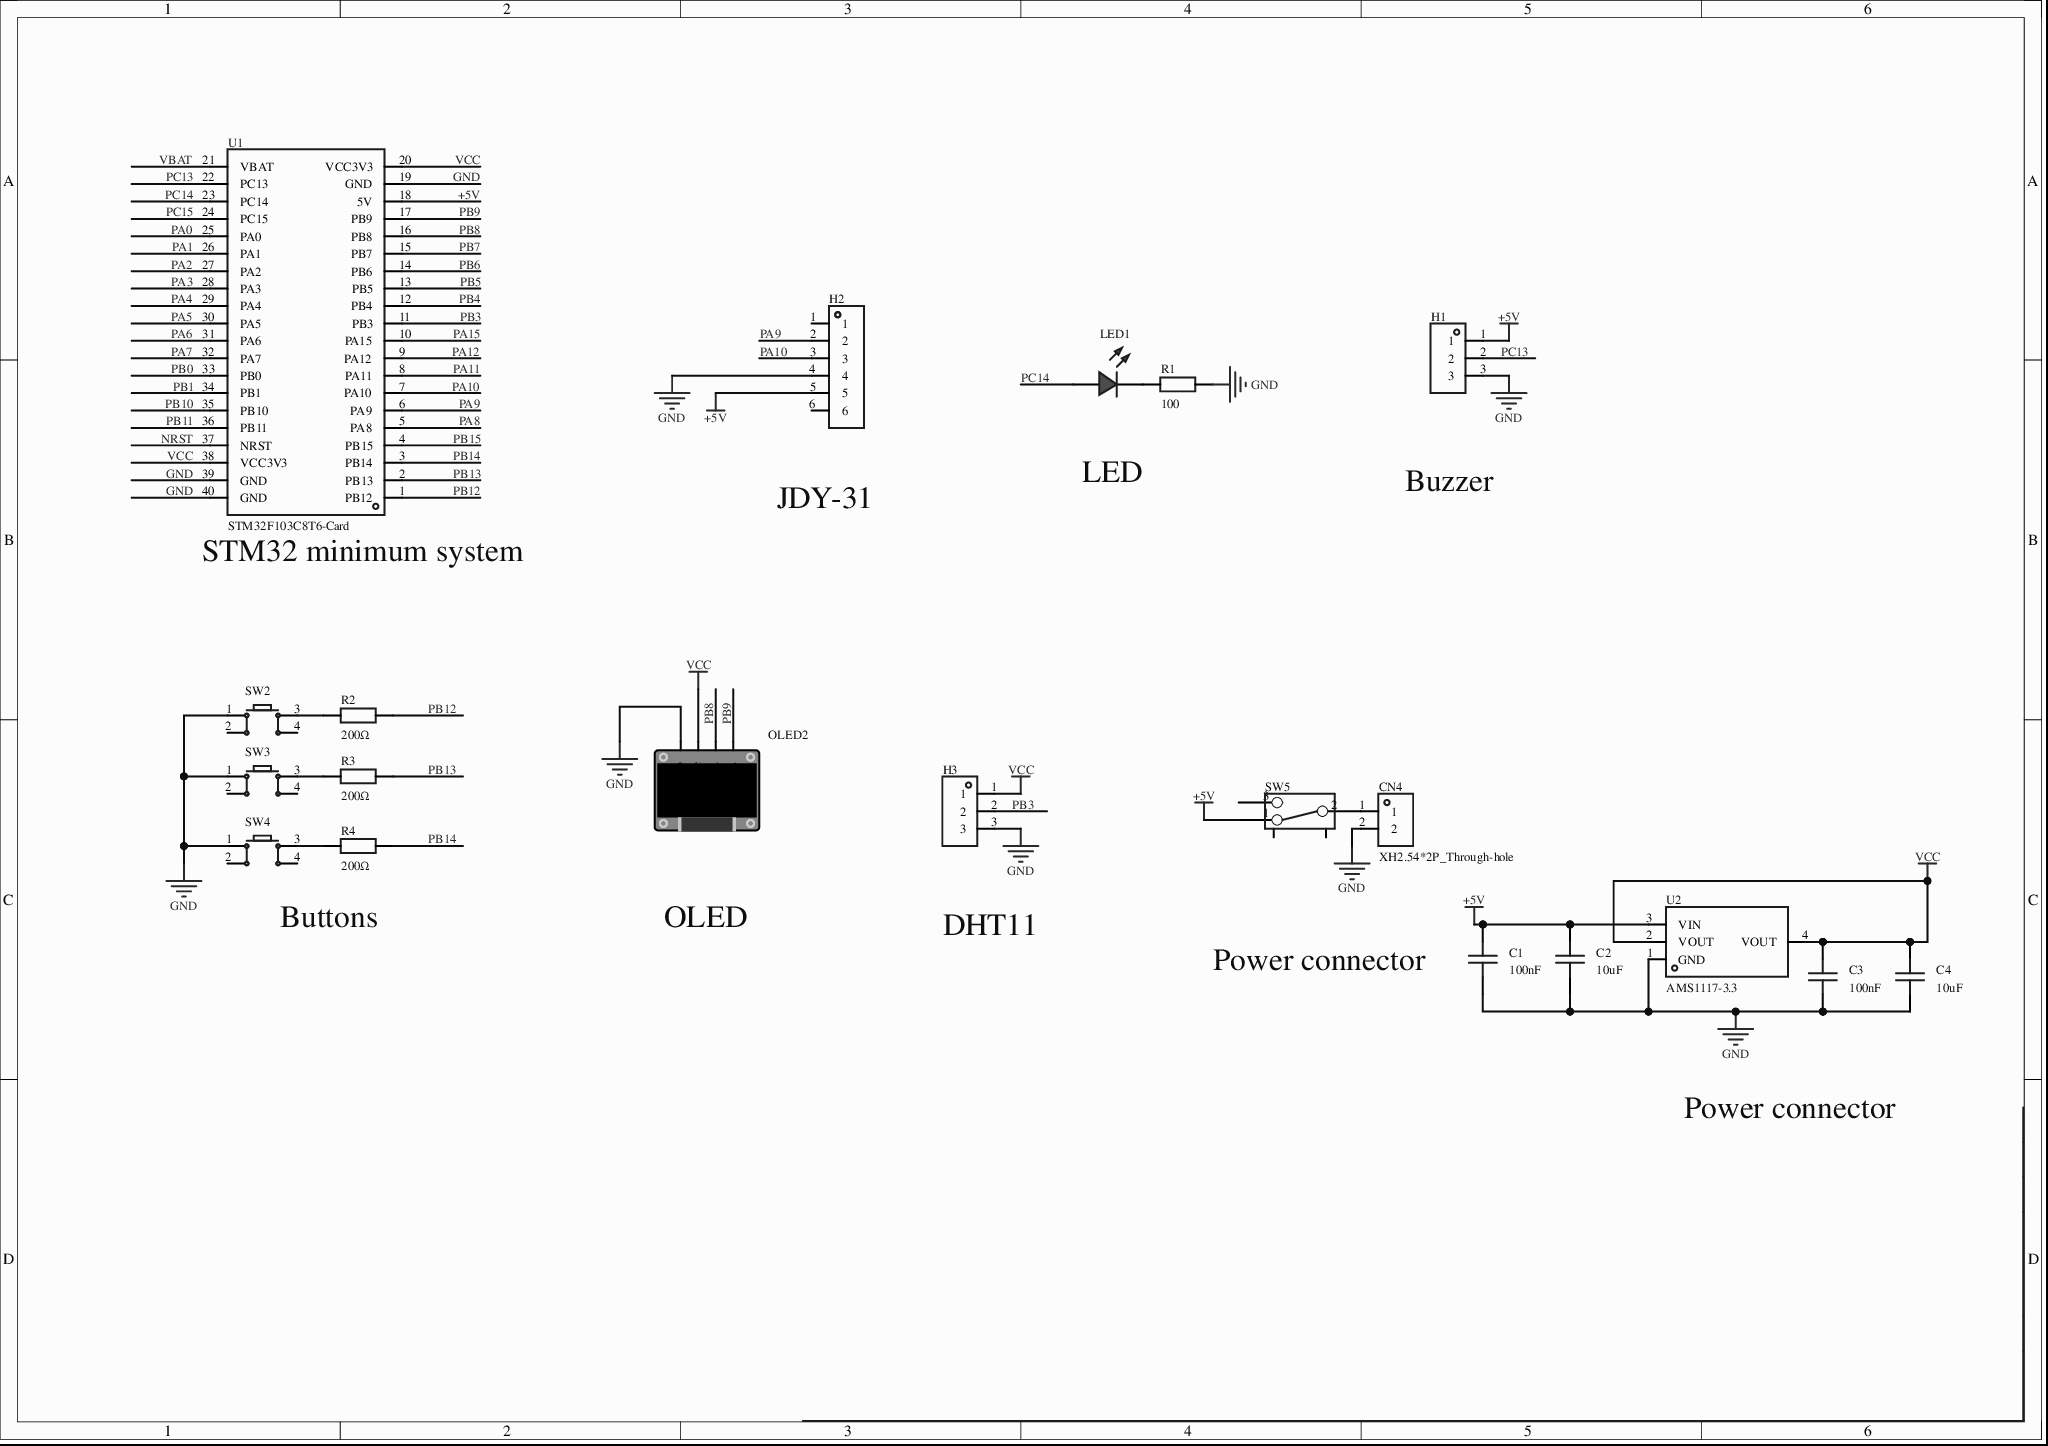
[diagram p0: MISC51821-3.schdoc]
# Altium project MISC51821-2.PrjPcb
1 sheet, 20 parts. Net scope: global (net labels, ports and power ports of the same name join across sheets).
Board file: MISC51821.pcbdoc

## Sheet MISC51821-3.schdoc
size 297 x 209 mm; Version: V1.0; @Project Name: MISC51821; @Page Count: 1; @Update Date: 2026-04-25; @Create Date: 2026-04-25; @Schematic Name: MISC51821; @Page No: 1; @Create Time: 23:22:16; @Update Time: 17:32:40; @Board Name: MISC51821

### Parts
C1  100nF  [C0603]
C2  10uF  [C0603]
C3  100nF  [C0603]
C4  10uF  [C0603]
CN4  XH2.54*2P_Through-hole  [CONN-TH_2P-P2.50-XH2.54-2P]
H1  (no value)  [HDR-TH_3P-P2.54-V-F]
H2  (no value)  [HDR-TH_6P-P2.54-V-F]
H3  (no value)  [HDR-TH_3P-P2.54-V-F]
LED1  (no value)  [LED_TH-3mm]
OLED2  (no value)  [0.96OLED_4P]
R1  100  [Res_1/8W]
R2  200Ω  [Res_1/8W]
R3  200Ω  [Res_1/8W]
R4  200Ω  [Res_1/8W]
SW2  (no value)  [SW-TH_4P-L6.0-W6.0-P4.50-LS6.5]
SW3  (no value)  [SW-TH_4P-L6.0-W6.0-P4.50-LS6.5]
SW4  (no value)  [SW-TH_4P-L6.0-W6.0-P4.50-LS6.5]
SW5  (no value)  [拨动开关]
U1  STM32F103C8T6-Card  [CONN-TH_L53.3-W22.9_STM32F103C8T6-CARD]
U2  AMS1117-3.3  [SOT-223-3_L6.5-W3.4-P2.30-LS7.0-BR]

### Nets
+5V: C1.2 C2.2 H1.1 H2.5 SW5.1 U1.18(5V) U2.3(VIN)
GND: C1.1 C2.1 C3.1 C4.1 CN4.2 H1.3 H2.4 H3.3 OLED2.1(GND) R1.2 SW2.1 SW3.1 SW4.1 U1.19(GND) U1.39(GND) U1.40(GND) U2.1(GND)
VCC: C3.2 C4.2 H3.1 OLED2.2(VCC) U1.20(VCC3V3) U1.38(VCC3V3) U2.2(VOUT) U2.4(VOUT)
NRST: U1.37(NRST)
PA0: U1.25(PA0)
PA1: U1.26(PA1)
PA2: U1.27(PA2)
PA3: U1.28(PA3)
PA4: U1.29(PA4)
PA5: U1.30(PA5)
PA6: U1.31(PA6)
PA7: U1.32(PA7)
PA8: U1.5(PA8)
PA9: H2.2 U1.6(PA9)
PA10: H2.3 U1.7(PA10)
PA11: U1.8(PA11)
PA12: U1.9(PA12)
PA15: U1.10(PA15)
PB0: U1.33(PB0)
PB1: U1.34(PB1)
PB3: H3.2 U1.11(PB3)
PB4: U1.12(PB4)
PB5: U1.13(PB5)
PB6: U1.14(PB6)
PB7: U1.15(PB7)
PB8: OLED2.3(SCL) U1.16(PB8)
PB9: OLED2.4(SDA) U1.17(PB9)
PB10: U1.35(PB10)
PB11: U1.36(PB11)
PB12: R2.2 U1.1(PB12)
PB13: R3.2 U1.2(PB13)
PB14: R4.2 U1.3(PB14)
PB15: U1.4(PB15)
PC13: H1.2 U1.22(PC13)
PC14: LED1.1(C) U1.23(PC14)
PC15: U1.24(PC15)
VBAT: U1.21(VBAT)
NetCN4_1: CN4.1 SW5.2
NetLED1_2: LED1.2(A) R1.1
NetR2_1: R2.1 SW2.3
NetR3_1: R3.1 SW3.3
NetR4_1: R4.1 SW4.3

Not connected (* = marked no-connect by the designer): H2 1 6; SW2 2 4; SW3 2 4; SW4 2 4; SW5 3 4 5

### Notes on the sheet
- 主控：
  STM32F103C8T6
  晶振电路
  复位电路
  串口：
  JDY-31  		PA9，PA10 	(串口1）
  GPIO:
  LED灯	PC14
  蜂鸣器  PC13
  按键：	PB12设置键，PB13加键，PB14减键，
  按键加电阻不用太大200Ω
  IIC:
  0.96英寸OLED显示屏	PB8，PB9
  One-Wire:
  DHT11  PB3
  供电：通过AMS1117-3.3V线性稳压芯片转换为3.3V
- JDY-31
- LED
- Buzzer
- (near U1) STM32 minimum system
- Buttons
- OLED
- DHT11
- (near C1) Power connector
- Power connector

### Library data of the parts
C1-C4 = CAP_0603: Symbol: Capacitance; ConvertToPcb: yes; ModelId: ac125912035d415993ca9572d50418b10819f05c4eef4c71ace90d822a990e87; ModelName: C0603_L1.6-W0.8-H0.8; ModelTransform: 62.992,31.496,0,0,0,0,0,0,0; Device: CAP_0603; AddInBom: yes; Supplier Footprint: 0603; FootprintName: C0603
  C1 C3: Value: 100nF
  C2 C4: Value: 10uF
CN4 = XH2.54*2P_直插: 3D Model: 325c595e30db4df8abe76612dd40b0fa0819f05c4eef4c71ace90d822a990e87; 3D Model Transform: 295.275,228.346,0,180,0,0,-0.002,-20.079,-137.795; AddInBom: yes; Device: XH2.54*2P_Through-hole; Symbol: XH2.54*2P_Through-hole; LCSC Part Name: XH2.54*2P_直插; Supplier Part: C9900008615; Manufacturer Part: XH2.54*2P_直插; Supplier Footprint: XH2.54_2P; JLCPCB Part Class: Extended Part; Supplier: LCSC; FootprintName: CONN-TH_2P-P2.50-XH2.54-2P; ConvertToPcb: yes; ModelName: CONN-TH_2P-P2.50-XH2.54-2P
H1 H3 = HDR-F_2.54_1x3P: Symbol: PM254V-11-03-H85; 3D Model: f3b3cc5aae9641bf9e56fc160cef875b; 3D Model Transform: 299.9994,100,0,0,0,0,0,0,-118.11; ConvertToPcb: yes; ModelName: HDR2.54-F-LI-1X3P; Device: HDR-F_2.54_1x3P; Supplier Part: C541850; Supplier Footprint: 插件; FootprintName: HDR-TH_3P-P2.54-V-F; AddInBom: yes
H2 = HDR-F_2.54_1x6P: Symbol: Header-Female-2.54_1x6; ConvertToPcb: yes; ModelId: 0f5bcf94dcda47d085f24cdca1696fe9; ModelTransform: 619.684,94.488,0,0,0,0,0,0,-125.984; Device: HDR-F_2.54_1x6P; AddInBom: yes; SupplierPart: C40877; Supplier Footprint: 插件; FootprintName: HDR-TH_6P-P2.54-V-F; ModelName: HDR-TH_6P-P2.54-V-F
LED1 = LED_TH-R_3mm: ConvertToPcb: yes; ModelId: a497c992633541038a38947cdc58012f0819f05c4eef4c71ace90d822a990e87; ModelName: LED-TH-3mm_R; ModelTransform: 141.274,153.327,0,0,0,0,-5.984,0,-137.795; Symbol: LED_TH-R; Device: LED_TH-R_3mm; AddInBom: yes; FootprintName: LED_TH-3mm; Supplier Footprint: 插件
OLED2 = 0.96OLED模块_4P: Symbol: 0.96OLED module_4P; ConvertToPcb: yes; ModelId: 79c000fdb68d45a296c2e9bedf4f9055; ModelTransform: 1393.69792,1318.895,0,0,0,0,0,-560.079,-137.795; Device: 0.96OLED module_4P; AddInBom: yes; FootprintName: 0.96OLED_4P; Supplier Footprint: 插件; ModelName: 0.96OLED_4P
R1 = Res_AXIAL-1/8W: Symbol: Resistor; ConvertToPcb: yes; ModelId: b2b5ae7ae4c642178fe0039925c86a3f0819f05c4eef4c71ace90d822a990e87; ModelName: RES-TH_BD1.8-L3.2-P7.20-D0.4; ModelTransform: 282.86,66.88,253.09,0,0,0,0,0,-191; Device: Res_AXIAL-1/8W; Value: 100; AddInBom: yes; Supplier Footprint: 轴向引线; FootprintName: Res_1/8W
R2-R4 = Res_AXIAL-1/8W: Symbol: Resistor; 3D Model: b2b5ae7ae4c642178fe0039925c86a3f0819f05c4eef4c71ace90d822a990e87; 3D Model Transform: 282.86,66.88,253.09,0,0,0,0,0,-191; ConvertToPcb: yes; ModelName: RES-TH_BD1.8-L3.2-P7.20-D0.4; Device: Res_AXIAL-1/8W; Supplier Footprint: 轴向引线; Value: 200Ω; AddInBom: yes; FootprintName: Res_1/8W
SW2-SW4 = Key_TH_6x6x6: Contact current:50mA;Rated voltage(DC):12V;Insulation resistance:100MΩ;Circuit structure:SPST;Mounting:Through-hole;Button shape:Round button;Button/cap colour:Black;Actuation force:260gf@±30gf;Operating temperature:-25℃~+70℃;Pin style:PC pin;Switch length:6mm;Switch width:6mm;Switch height:6mm;With bracket:No;; Symbol: Tactile switch; AddInBom: yes; ModelId: 20eee248bc684ccd8cbdbb1d0d91ec6f0819f05c4eef4c71ace90d822a990e87; ModelName: SW-TH_4P-L6.0-W6.0-H5.0-LS6.5-P4.50; ModelTransform: 236.22,323.03,0,90,0,0,0,0,-137.795; Device: Key_TH_6x6x6; FootprintName: SW-TH_4P-L6.0-W6.0-P4.50-LS6.5; ConvertToPcb: yes; Supplier Footprint: 插件
SW5 = 拨动开关_正: Device: Toggle switch_positive; Symbol: Toggle switch; ConvertToPcb: yes; ModelId: 4321fe59a4074cbfb4989553f297c68f0819f05c4eef4c71ace90d822a990e87; ModelName: SW-TH_SS-12D02-VG4; ModelTransform: 370.09,208.7,472.35,0,0,0,0,0,-110; FootprintName: Toggle switch; AddInBom: yes; Supplier Footprint: 插件
U1 = STM32F103C8T6-Card: AddInBom: yes; Device: STM32F103C8T6-Card; Symbol: STM32F103C8T6-CARD; FootprintName: CONN-TH_L53.3-W22.9_STM32F103C8T6-CARD; LCSC Part Name: STM32F103C8T6-Card; SupplierPart: C9900077949; ManufacturerPart: STM32F103C8T6-Card; Supplier Footprint: 插件; Supplier: LCSC; ConvertToPcb: yes
U2 = AMS1117-3.3_C6186: Output type:Fixed;Operating voltage:-;Output voltage:3.3V;Output current:1A;Power supply ripple rejection ratio(PSRR):72dB@(120Hz);Output polarity:Positive;; Manufacturer: AMS; AddInBom: yes; ModelId: 925194bf9823436183a3e0b978a8d076; ModelName: SOT-223-4P_L6.5-W3.5-H1.6-LS7.0-P2.30; ModelTransform: 279.89794,255.905,0,180,0,0,-3.9385,-0.0005,0; Output Type: Fixed; Output Voltage: 3.3V; Output Current: 1A; Voltage Dropout: 1.3V@(800mA); Number of Outputs: 1; Symbol: AMS1117-3.3; Device: AMS1117-3.3_C6186; LCSC Part Name: 输出3.3V 1A; SupplierPart: C6186; ManufacturerPart: AMS1117-3.3; Supplier Footprint: SOT-223; Datasheet: https://atta.szlcsc.com/upload/public/pdf/source/20180727/C6186_7A095716F0823C02F1997A905E26C086.pdf; Supplier: LCSC; ConvertToPcb: yes; FootprintName: SOT-223-3_L6.5-W3.4-P2.30-LS7.0-BR; Voltage - Supply: -; Power Supply Rejection Ratio (PSRR): 72dB@(120Hz); standby current: -; Noise: -; Features: Overcurrent protection(OCP); Thermal shutdown(TSD); Operating Temperature: -; Output Configuration: Positive